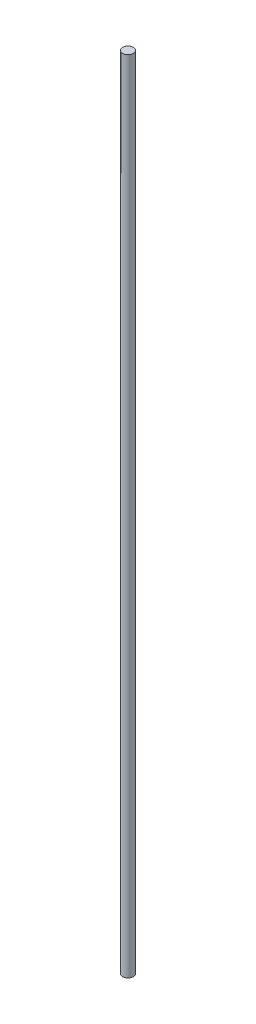
from build123d import *

# Parameters (mm, degrees)
SKETCH1_R           = 4
BOSS_EXTRUDE1_DEPTH = 600


with BuildPart() as part:
    # Sketch1 → Boss-Extrude1 (new body)
    with BuildSketch(Plane(origin=(0, 0, 0), x_dir=(1, 0, 0), z_dir=(0, 1, 0))):
        with Locations(Location((0, 0, 0), (0, 0, 270))):
            Circle(SKETCH1_R)
    extrude(amount=BOSS_EXTRUDE1_DEPTH)


solid = part.part
